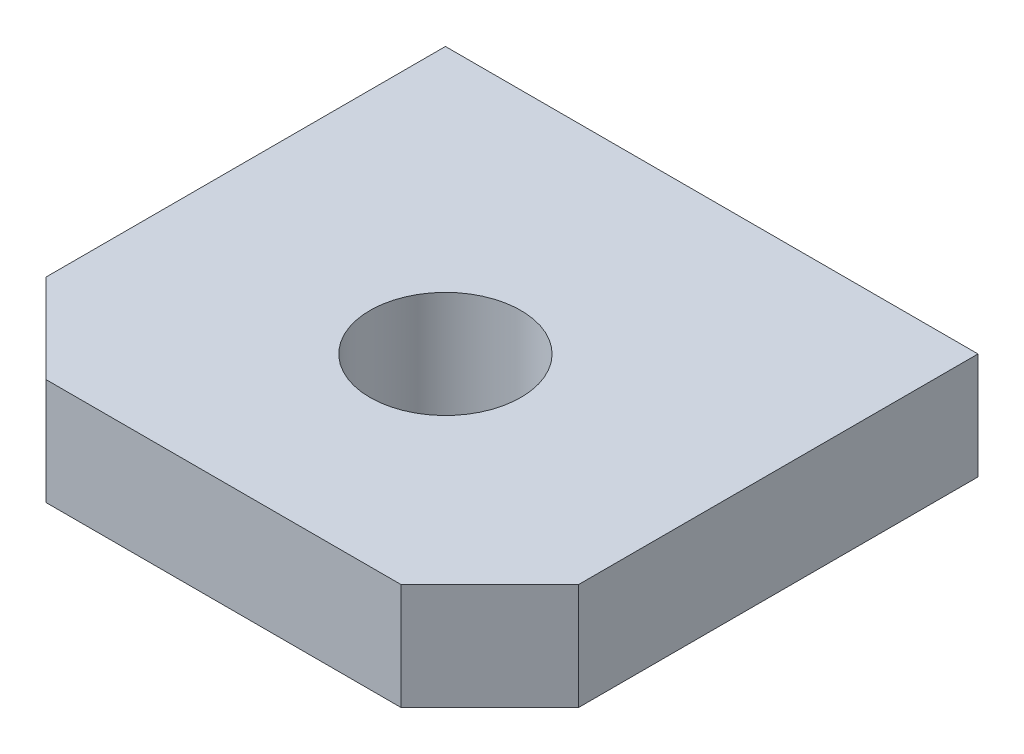
SolidWorks part; units mm, degrees
material "1023 碳钢板 (SS)"
ref_plane "Front Plane" through (0, 0, 0) normal (0, 0, 1) x (1, 0, 0)
ref_plane "Top Plane" through (0, 0, 0) normal (0, 1, 0) x (1, 0, 0)
ref_plane "Right Plane" through (0, 0, 0) normal (1, 0, 0) x (0, 0, -1)
sketch "Sketch1" plane through (0, 0, 0) normal (0, 1, 0) x (1, 0, 0)
  line L0 (30, -55) -> (30, 0) construction
  line L1 (0, 0) -> (60, 0)
  line L2 (0, 0) -> (0, -55)
  line L3 (0, -55) -> (60, -55)
  line L4 (60, 0) -> (60, -55)
  circle A0 centre (30, -30) radius 8.5
  dimension "D3" = 17
  dimension "D1" = 60
  dimension "D2" = 55
  dimension "D4" = 25
extrude "Boss-Extrude1" add sketch "Sketch1" along normal blind 12
chamfer "Chamfer1" distance 10 angle 45 2 edges at (60, 6, 55) (0, 6, 55)
